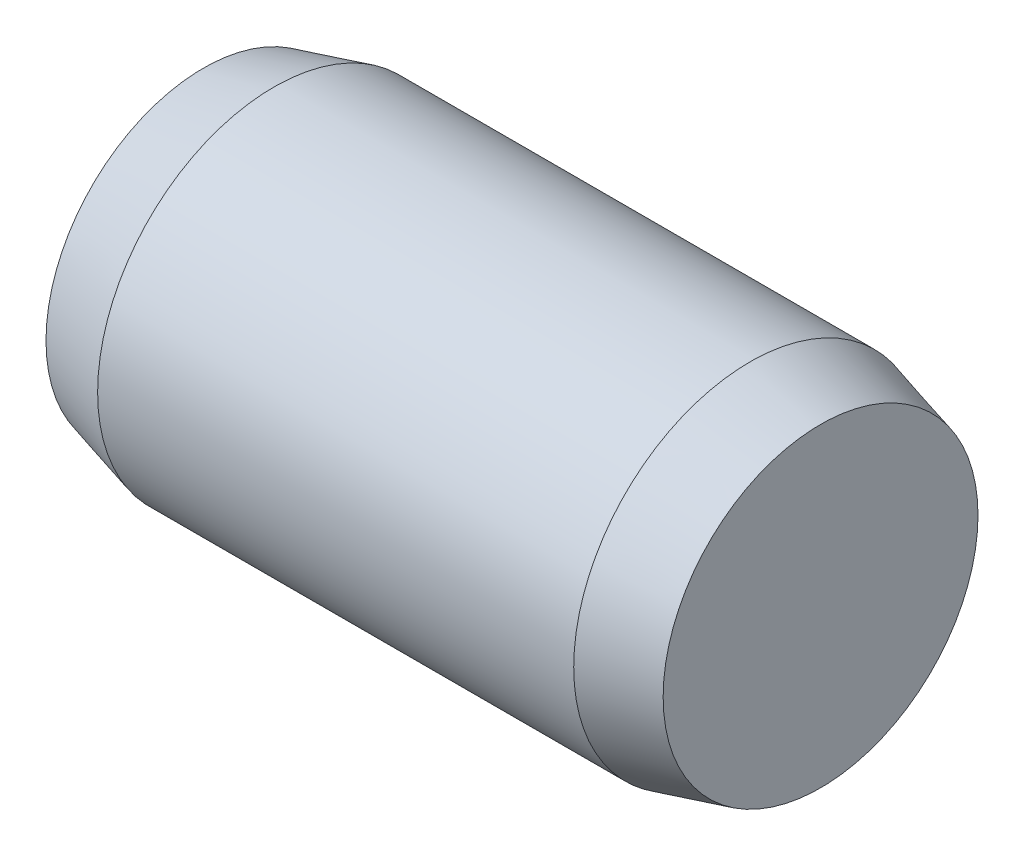
from build123d import *


with BuildPart() as part:
    # Sketch1 → Base-Revolve (revolve)
    with BuildSketch(Plane.XY, mode=Mode.PRIVATE) as base_revolve_sk:
        Polygon((0, 0), (14, 0), (14, 3.571281292), (12.4, 4), (1.6, 4), (0, 3.571281292), align=None)
    revolve(base_revolve_sk.sketch.rotate(Axis((-1.655717266, 0, 0), (1, 0, 0)), 90), axis=Axis((-1.655717266, 0, 0), (1, 0, 0)))


solid = part.part
